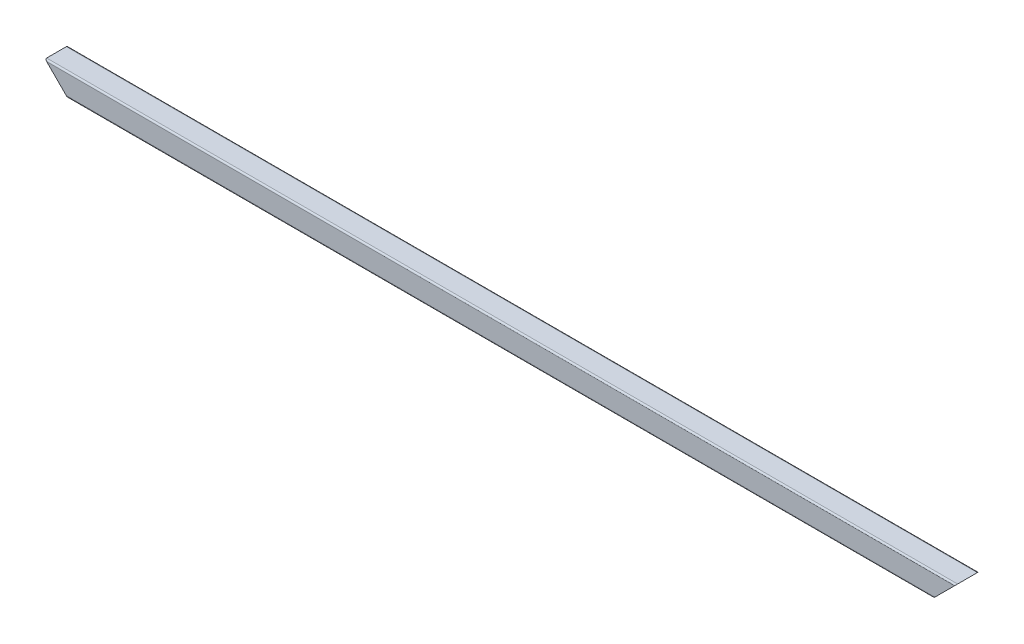
SolidWorks part; units mm, degrees
ref_plane "前视基准面" through (0, 0, 0) normal (0, 0, 1) x (1, 0, 0)
ref_plane "上视基准面" through (0, 0, 0) normal (0, 1, 0) x (1, 0, 0)
ref_plane "右视基准面" through (0, 0, 0) normal (1, 0, 0) x (0, 0, -1)
sketch "草图1" plane through (0, 0, 0) normal (0, 0, 1) x (1, 0, 0)
  line L0 (-3000, 0) -> (3000, 0)
  point P4 (0, 0)
  dimension "D1" = 6000
other "Gb／6728-1986方形空心型钢 150 X 150 X 5(1)"
ref_plane "基准面1" through (-3000, 0, 0) normal (1, 0, 0) x (0, 1, 0)
sketch "Sketch1" plane through (-3000, 0, 0) normal (1, 0, 0) x (0, 1, 0)
  line L0 (-65, -70) -> (65, -70)
  line L1 (-70, -65) -> (-70, 65)
  line L2 (65, 70) -> (-65, 70)
  line L3 (70, 65) -> (70, -65)
  line L4 (-65, -75) -> (65, -75)
  line L5 (-75, -65) -> (-75, 65)
  line L6 (65, 75) -> (-65, 75)
  line L7 (75, 65) -> (75, -65)
  arc A0 (75, 65) -> (65, 75) centre (65, 65) ccw
  arc A1 (65, -75) -> (75, -65) centre (65, -65) ccw
  arc A2 (-75, -65) -> (-65, -75) centre (-65, -65) ccw
  arc A3 (-65, 75) -> (-75, 65) centre (-65, 65) ccw
  arc A4 (-65, 70) -> (-70, 65) centre (-65, 65) ccw
  arc A5 (70, 65) -> (65, 70) centre (65, 65) ccw
  arc A6 (65, -70) -> (70, -65) centre (65, -65) ccw
  arc A7 (-70, -65) -> (-65, -70) centre (-65, -65) ccw
  point P0 (-75, 0)
  point P1 (75, 0)
  point P2 (0, 75)
  point P3 (0, -75)
  point P4 (0, 0)
  point P5 (-75, -75)
  point P6 (75, -75)
  point P7 (75, 75)
  point P8 (-75, 75)
  point P33 (0, 0)
  dimension "D1" = 10
  dimension "Thickness" = 5
  dimension "V_leg" = 150
sketch "草图6" plane through (0, 0, -75) normal (0, 0, -1) x (-1, 0, 0)
  line L0 (3000, 75) -> (3000, -75)
  line L1 (3000, -75) -> (2850, -75)
  line L2 (-3000, -75) -> (3000, -75) construction
  line L3 (2850, -75) -> (3000, 75)
  line L4 (0, 0) -> (0, -789.7314) construction
  line L5 (-2850, -75) -> (-3000, 75)
  line L6 (-3000, -75) -> (-2850, -75)
  line L7 (-3000, 75) -> (-3000, -75)
extrude "切除-拉伸1" cut sketch "草图6" against normal through all
